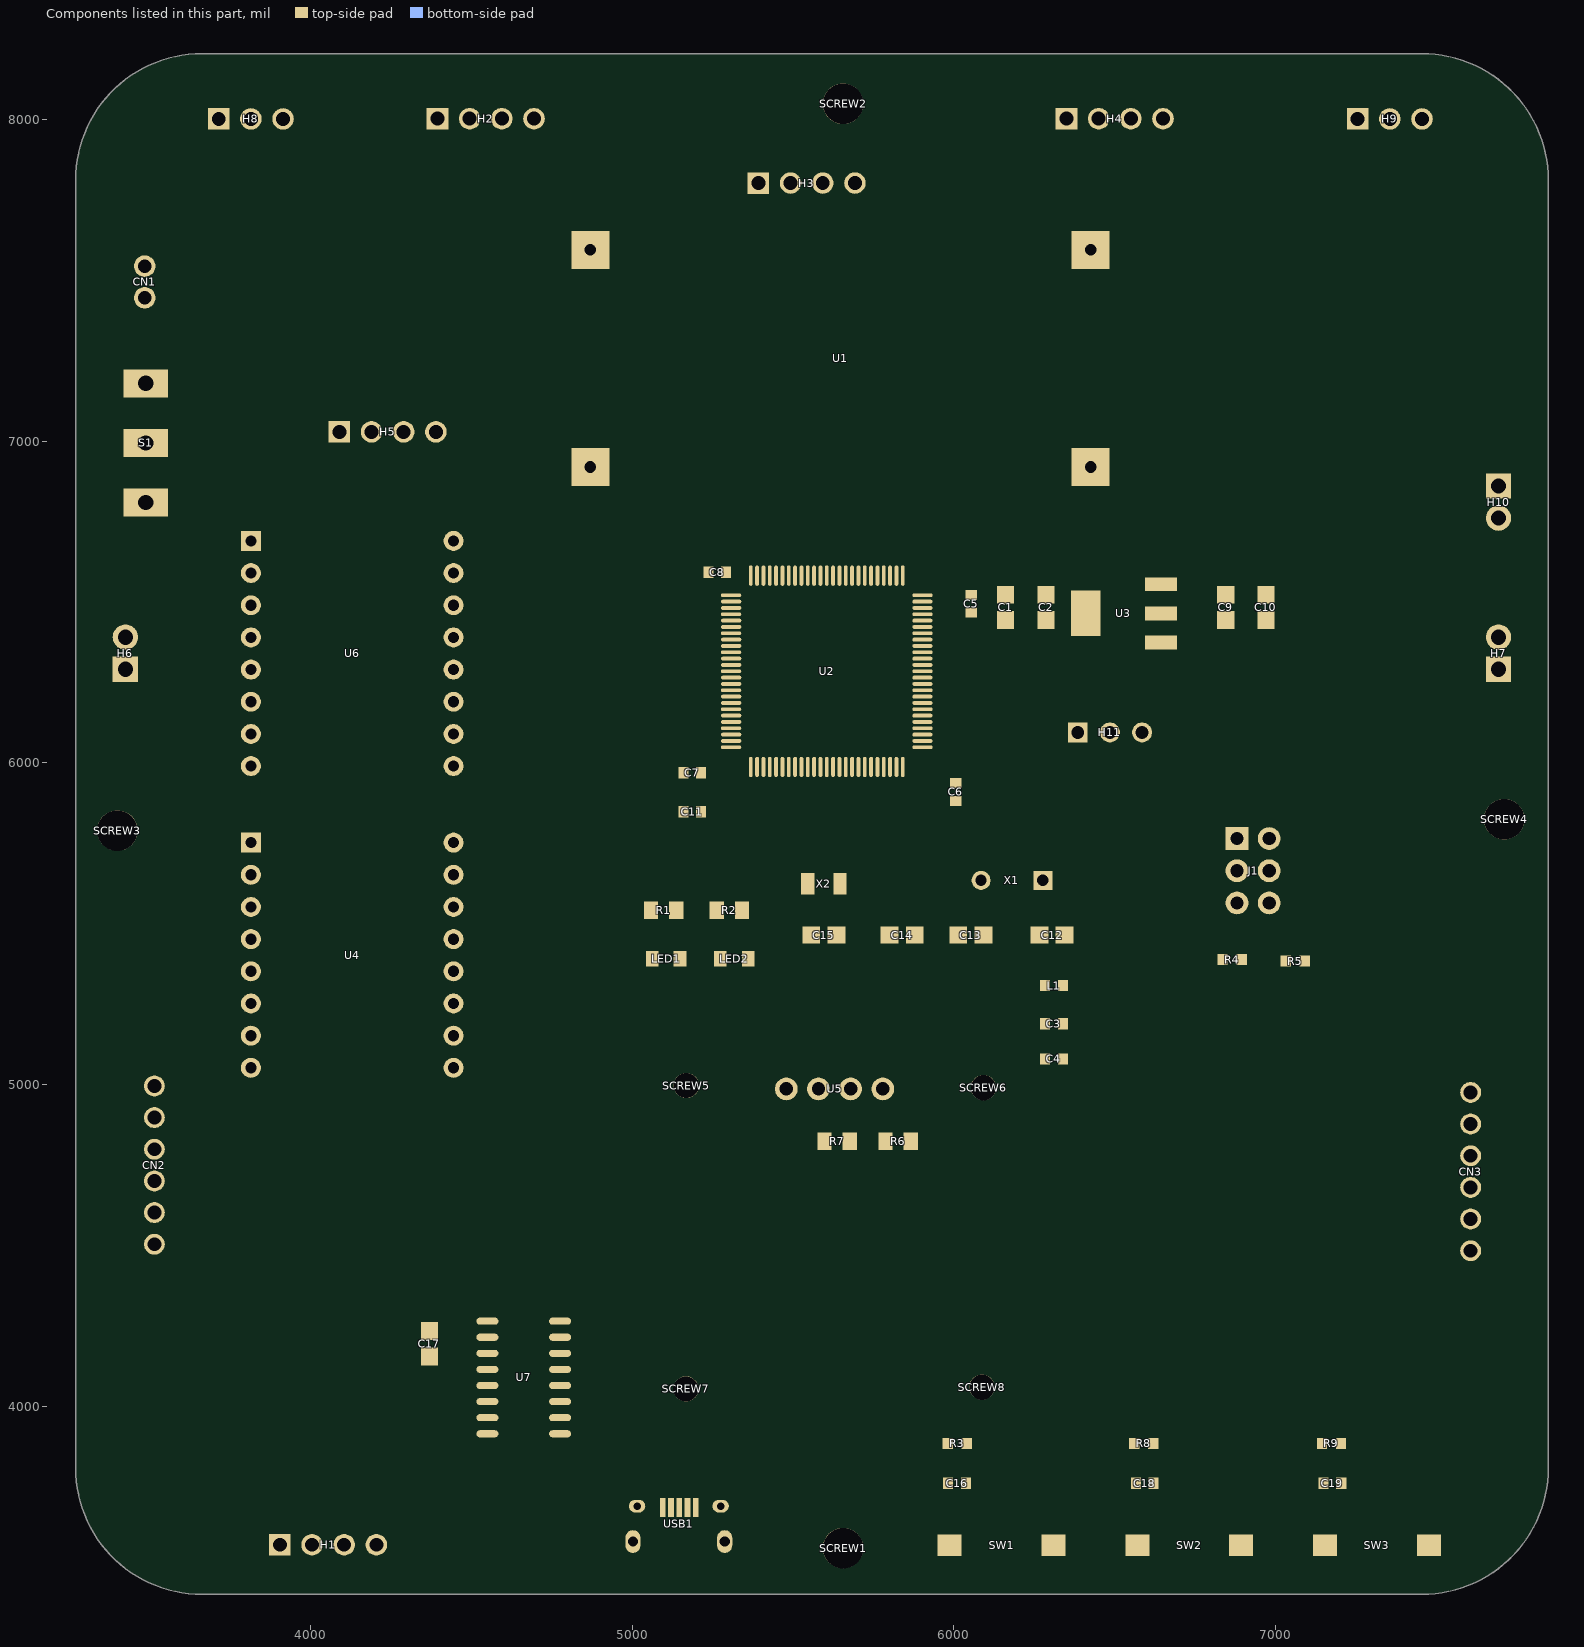
[diagram p0: the components of this part, seen from the top]
# Altium PCB MISC62445.pcbdoc (part 3 of 3)
Units mil, origin at the board's own origin, x right, y up, seen from the top; angles counter-clockwise.
Board outline 4577.56 x 4789.41 mil, 2 copper layers (Top Layer, Bottom Layer), stack 62.206 mil thick; 68 components, 65 nets, 307 pads, 204 vias.

## Silkscreen, mask and mechanical layers (free items; w line width, h text height)
Top Silkscreen Layer:
  text "3.3V" at 4365,8065 h30
  text "Trig_L" at 4450,8065 h30
  text "Echo_L" at 4555,8065 h30
  text "GND" at 4670,8065 h30
  text "3.3V" at 6315,8065 h30
  text "Trig_R" at 6400,8065 h30
  text "Echo_R" at 6505,8065 h30
  text "GND" at 6620,8065 h30
  text "PA1" at 7220,8065 h50
  text "5V" at 7330,8065 h50
  text "GND" at 7425,8065 h50
  text "PA0" at 3675,8060 h50
  text "5V" at 3785,8060 h50
  text "GND" at 3880,8060 h50
  text "3.3V" at 5355,7865 h30
  text "Trig_M" at 5440,7865 h30
  text "Echo_M" at 5545,7865 h30
  text "GND" at 5660,7865 h30
  text "Right ultrasonic" at 6340,7850 h80
  text "Left ultrasonic" at 4395,7845 h80
  text "Left servo brush" at 3565,7825 h100
  text "Right servo brush" at 7115,7820 h100
  text "Middle ultrasonic" at 5745,7695 h80
  text "Battery connector" at 3320,7655 h80
  text "GND" at 3590,7505 h80
  text "12V" at 3590,7395 h80
  text "5V" at 4075,7090 h30
  text "GND" at 4165,7090 h30
  text "BT_TX" at 4255,7090 h30
  text "BT_RX" at 4360,7090 h30
  text "Bluetooth" at 4115,6850 h120
  text "PC16" at 7530,6835 h50
  text "GND" at 7551.98,6735 h50
  text "12V" at 3625,6660 h80
  text "Vacuum motor" at 7515,6615 h80
  text "FL+" at 3495,6350 h80
  text "FR+" at 7510,6346.71 h80
  text "FL-" at 3495,6245 h80
  text "FR-" at 7510,6241.71 h80
  text "PA2" at 6335,6160 h50
  text "3.3V" at 6435,6160 h50
  text "GND" at 6549.83,6160 h50
  text "Front left motor" at 3290,6130 h80
  text "Front right motor" at 7520,6125 h80
  text "Temp/humidity sensor" at 6250,5945 h80
  text "Boot mode" at 6780,5820 h80
  text "3.3V" at 6720,5740 h50
  text "3.3V" at 7040,5740 h50
  text "12V" at 3625,5715 h80
  text "GND" at 6745,5535 h50
  text "GND" at 7040,5535 h50
  text "PC13 LED" at 5255,5290 h50
  text "Power LED" at 4970,5288.66 h50
  text "BL+" at 3635,4965 h60
  text "BR-" at 7413.1,4950 h60
  text "GND" at 3640,4865 h60
  text "5V" at 7413.1,4850 h60
  text "AL" at 3640,4765 h60
  text "BR" at 7418.1,4750 h60
  text "BL" at 3640,4670 h60
  text "AR" at 7418.1,4655 h60
  text "5V" at 3640,4570 h60
  text "GND" at 7413.1,4555 h60
  text "BL-" at 3640,4470 h60
  text "BR+" at 7413.1,4455 h60
  text "Rear left motor" at 3355,4290 h80
  text "Rear right motor" at 7475,4270 h80
  text "PERSON_A" at 6635,4265 h130
  text "Reset button" at 6025,3650 h60
  text "OK button" at 6635,3650 h60
  text "Back button" at 7225,3650 h60
  text "SWD download" at 3780,3630 h60
  text "3.3V" at 3835,3460 h50
  text "SWIO" at 3945,3460 h50
  text "SWCLK" at 4060,3460 h50
  text "GND" at 4200,3460 h50